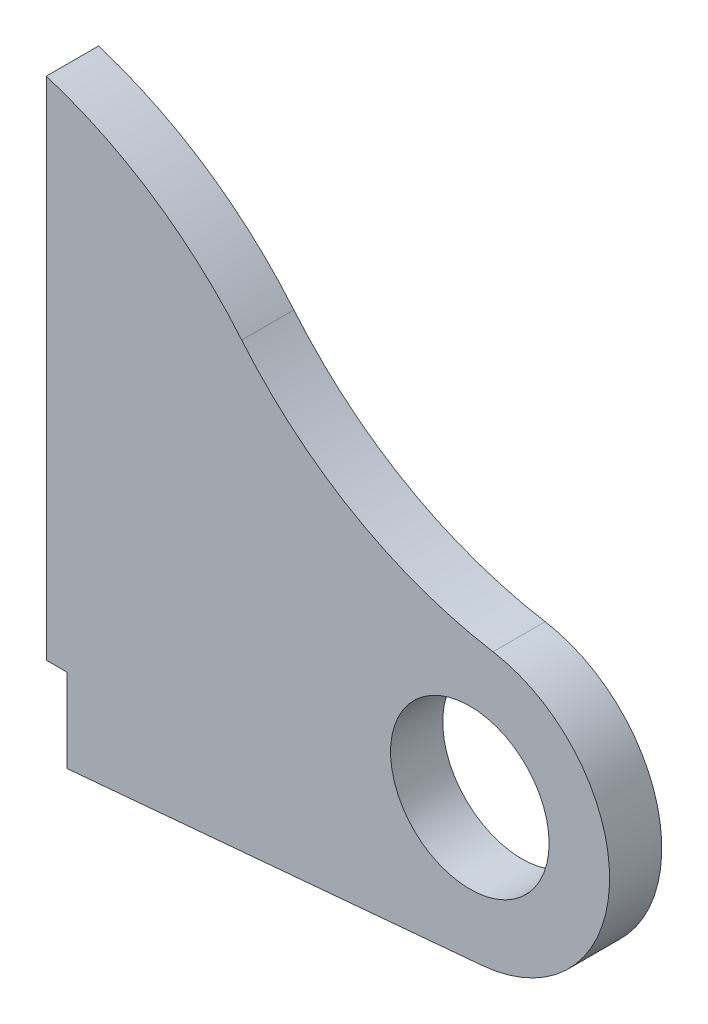
from build123d import *

# Parameters (mm, degrees)
SKETCH1_R           = 38
BOSS_EXTRUDE1_DEPTH = 25


with BuildPart() as part:
    # Sketch1 → Boss-Extrude1 (new body)
    with BuildSketch(Plane.XY):
        with BuildLine():
            Line((-203, 198), (-203, -44.5))
            Line((-203, -44.5), (-193, -44.5))
            Line((-193, -44.5), (-193, -84.5))
            Line((-193, -84.5), (5.958881534, -66.734486818))
            ThreePointArc((5.958881534, -66.734486818), (66.949661999, -2.596682146), (11.109877523, 66.072464926))
            ThreePointArc((11.109877523, 66.072464926), (-55.326905119, 89.868640022), (-109.363154487, 135.257931614))
            ThreePointArc((-109.363154487, 135.257931614), (-151.670232074, 173.361739233), (-203, 198))
        make_face()
        Circle(SKETCH1_R, mode=Mode.SUBTRACT)
    extrude(amount=BOSS_EXTRUDE1_DEPTH)


solid = part.part
